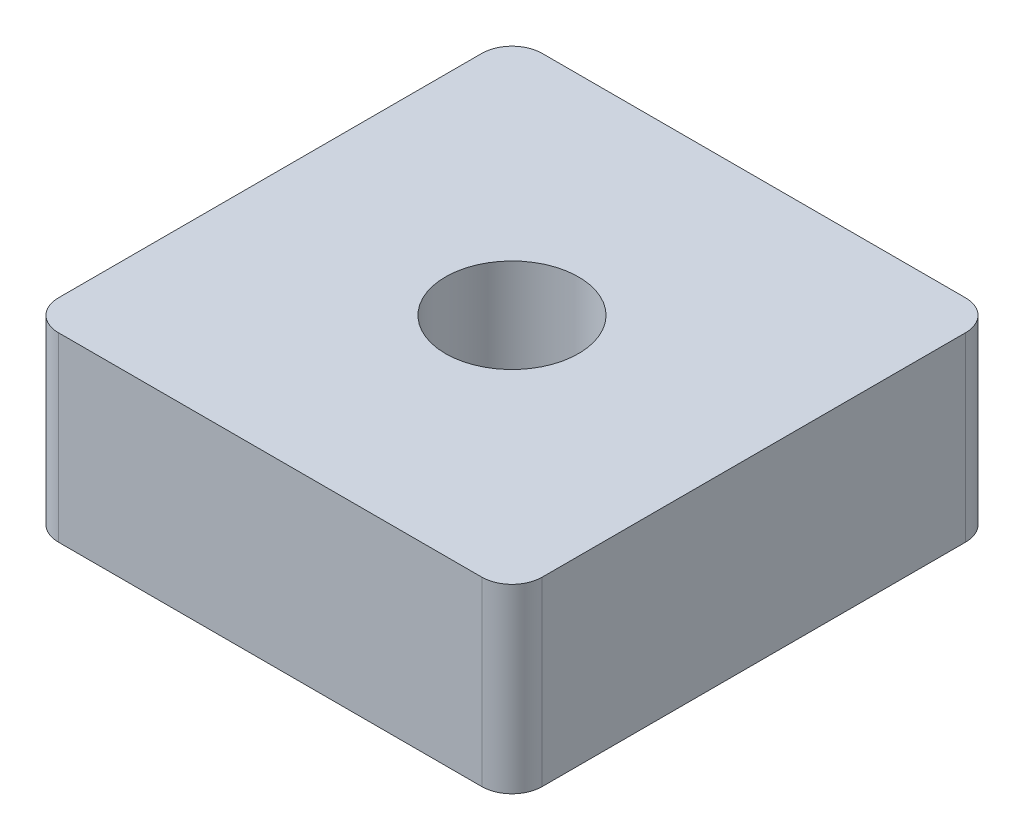
from build123d import *

# Parameters (mm, degrees)
SKETCH1_W              = 80
SKETCH1_H              = 80
BOSS_EXTRUDE1_DEPTH    = 30
FILLET1_R              = 5
M24X2_0_TAPPED_HOLE1_D = 22


with BuildPart() as part:
    # Sketch1 → Boss-Extrude1 (new body)
    with BuildSketch(Plane(origin=(0, 0, 0), x_dir=(1, 0, 0), z_dir=(0, 1, 0))):
        Rectangle(SKETCH1_W, SKETCH1_H)
    extrude(amount=BOSS_EXTRUDE1_DEPTH)

    # Fillet1
    fillet1_edges = [part.edges().sort_by_distance(p)[0] for p in [
        (40, 15, 40),
        (-40, 15, 40),
        (-40, 15, -40),
        (40, 15, -40),
    ]]
    fillet(fillet1_edges, radius=FILLET1_R)

    # M24x2.0 Tapped Hole1 (through all)
    with Locations(Plane(origin=(0, 30, 0), x_dir=(1, 0, 0), z_dir=(0, 1, 0))):
        with Locations((0, 0)):
            Hole(M24X2_0_TAPPED_HOLE1_D / 2)


solid = part.part
